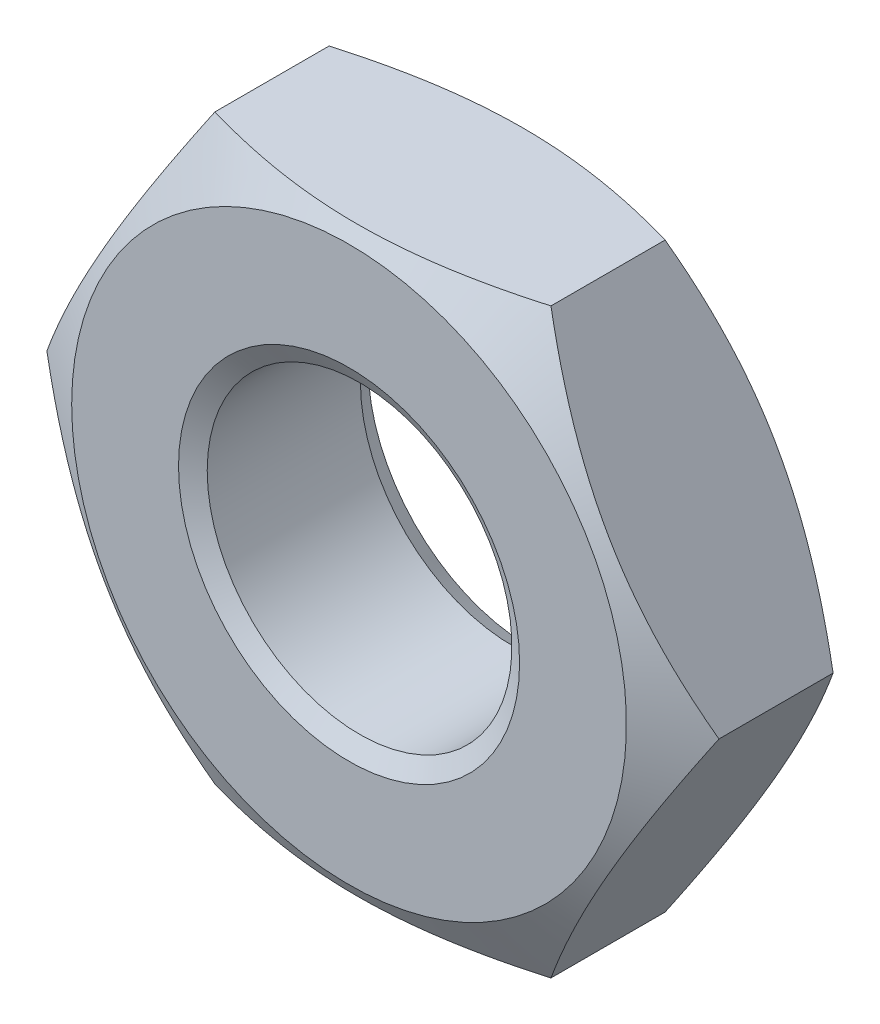
from build123d import *
from OCP.BRepFilletAPI import BRepFilletAPI_MakeChamfer

# Parameters (mm, degrees)
SKETCH1_R        = 4.188
BASENUT_DEPTH    = 5
ENDCHAMFER_SIZE  = 0.5
ENDCHAMFER_SIZE2 = 0.288675135


with BuildPart() as part:
    # Sketch1 → BaseNut (new body)
    with BuildSketch(Plane.XY):
        Polygon((4.618802154, -8), (9.237604307, 0), (4.618802154, 8), (-4.618802154, 8), (-9.237604307, 0), (-4.618802154, -8), align=None)
        Circle(SKETCH1_R, mode=Mode.SUBTRACT)
    extrude(amount=-BASENUT_DEPTH)

    # Sketch2 → Double-Chamfer (revolve, cut)
    with BuildSketch(Plane(origin=(0, 0, 0), x_dir=(1, 0, 0), z_dir=(0, 1, 0))):
        Polygon((-9.237604307, 5), (-7.625, 5), (-9.237604307, 4.068962469), align=None)
        Polygon((-9.237604307, 0.931037531), (-9.237604307, 0), (-7.625, 0), align=None)
    revolve(axis=Axis((0, 0, -3.375940562), (0, 0, 1)), mode=Mode.SUBTRACT)

    # EndChamfer: one chamfer whose edges measure the first distance from different faces: ONE call of the kernel's chamfer builder (chamfer() names one face for all edges)
    endchamfer_edges_1 = [part.edges().sort_by_distance(p)[0] for p in [
        (-4.188, 0, -5),
    ]]
    endchamfer_side_1 = [part.faces().sort_by_distance(p)[0] for p in [
        (-4.188, 0, -2.5),
    ]]
    endchamfer_edges_2 = [part.edges().sort_by_distance(p)[0] for p in [
        (-4.188, 0, 0),
    ]]
    endchamfer_side_2 = [part.faces().sort_by_distance(p)[0] for p in [
        (7.409332432, 0, 0),
    ]]
    endchamfer = BRepFilletAPI_MakeChamfer(part.part.solid().wrapped)
    for e in endchamfer_edges_1:
        endchamfer.Add(ENDCHAMFER_SIZE, ENDCHAMFER_SIZE2, e.wrapped, endchamfer_side_1[0].wrapped)  # the first distance lies on this face
    for e in endchamfer_edges_2:
        endchamfer.Add(ENDCHAMFER_SIZE, ENDCHAMFER_SIZE2, e.wrapped, endchamfer_side_2[0].wrapped)  # the first distance lies on this face
    add(Compound.cast(endchamfer.Shape()), mode=Mode.REPLACE)


solid = part.part
